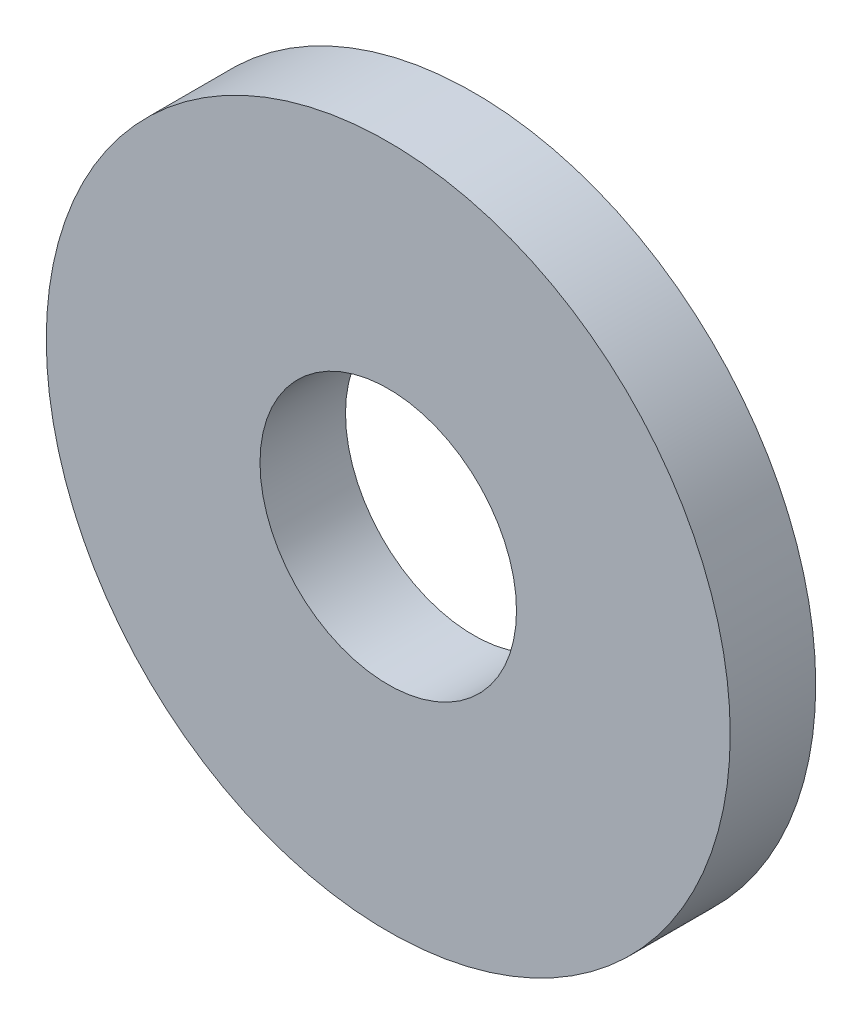
SolidWorks part; units mm, degrees
ref_plane "前视基准面" through (0, 0, 0) normal (0, 0, 1) x (1, 0, 0)
ref_plane "上视基准面" through (0, 0, 0) normal (0, 1, 0) x (1, 0, 0)
ref_plane "右视基准面" through (0, 0, 0) normal (1, 0, 0) x (0, 0, -1)
sketch "草图1" plane through (0, 0, 0) normal (0, 0, 1) x (1, 0, 0)
  circle A0 centre (0, 0) radius 3
  circle A1 centre (0, 0) radius 8
  dimension "D1" = 16
  dimension "D2" = 6
extrude "凸台-拉伸1" add sketch "草图1" along normal blind 2
